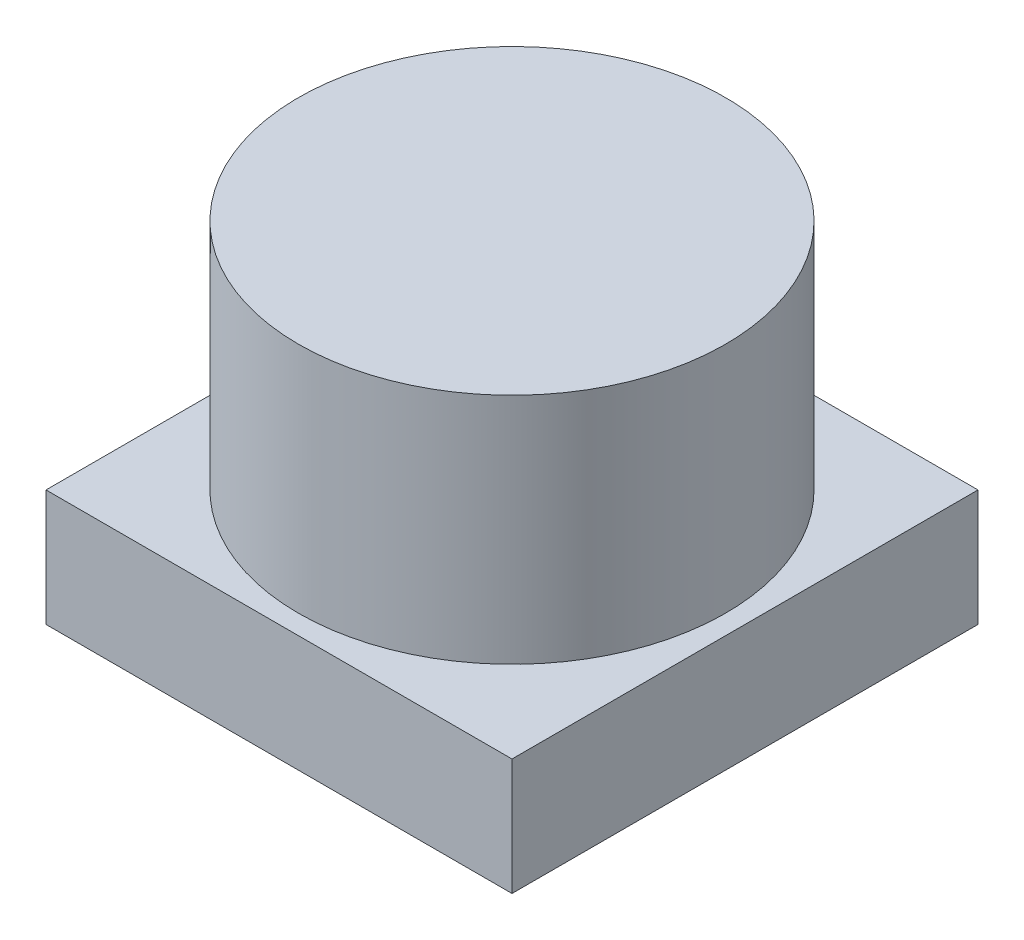
from build123d import *

# Parameters (mm, degrees)
SKETCH1_R           = 2.75
BOSS_EXTRUDE1_DEPTH = 3
SKETCH2_W           = 6
SKETCH2_H           = 6
BOSS_EXTRUDE2_DEPTH = 1.5


with BuildPart() as part:
    # Sketch1 → Boss-Extrude1 (new body)
    with BuildSketch(Plane(origin=(0, 0, 0), x_dir=(1, 0, 0), z_dir=(0, 1, 0))):
        with Locations(Location((0, 0, 0), (0, 0, 270))):
            Circle(SKETCH1_R)
    extrude(amount=BOSS_EXTRUDE1_DEPTH)

    # Sketch2 → Boss-Extrude2 (add)
    with BuildSketch(Plane.XZ):
        Rectangle(SKETCH2_W, SKETCH2_H)
    extrude(amount=BOSS_EXTRUDE2_DEPTH)


solid = part.part
